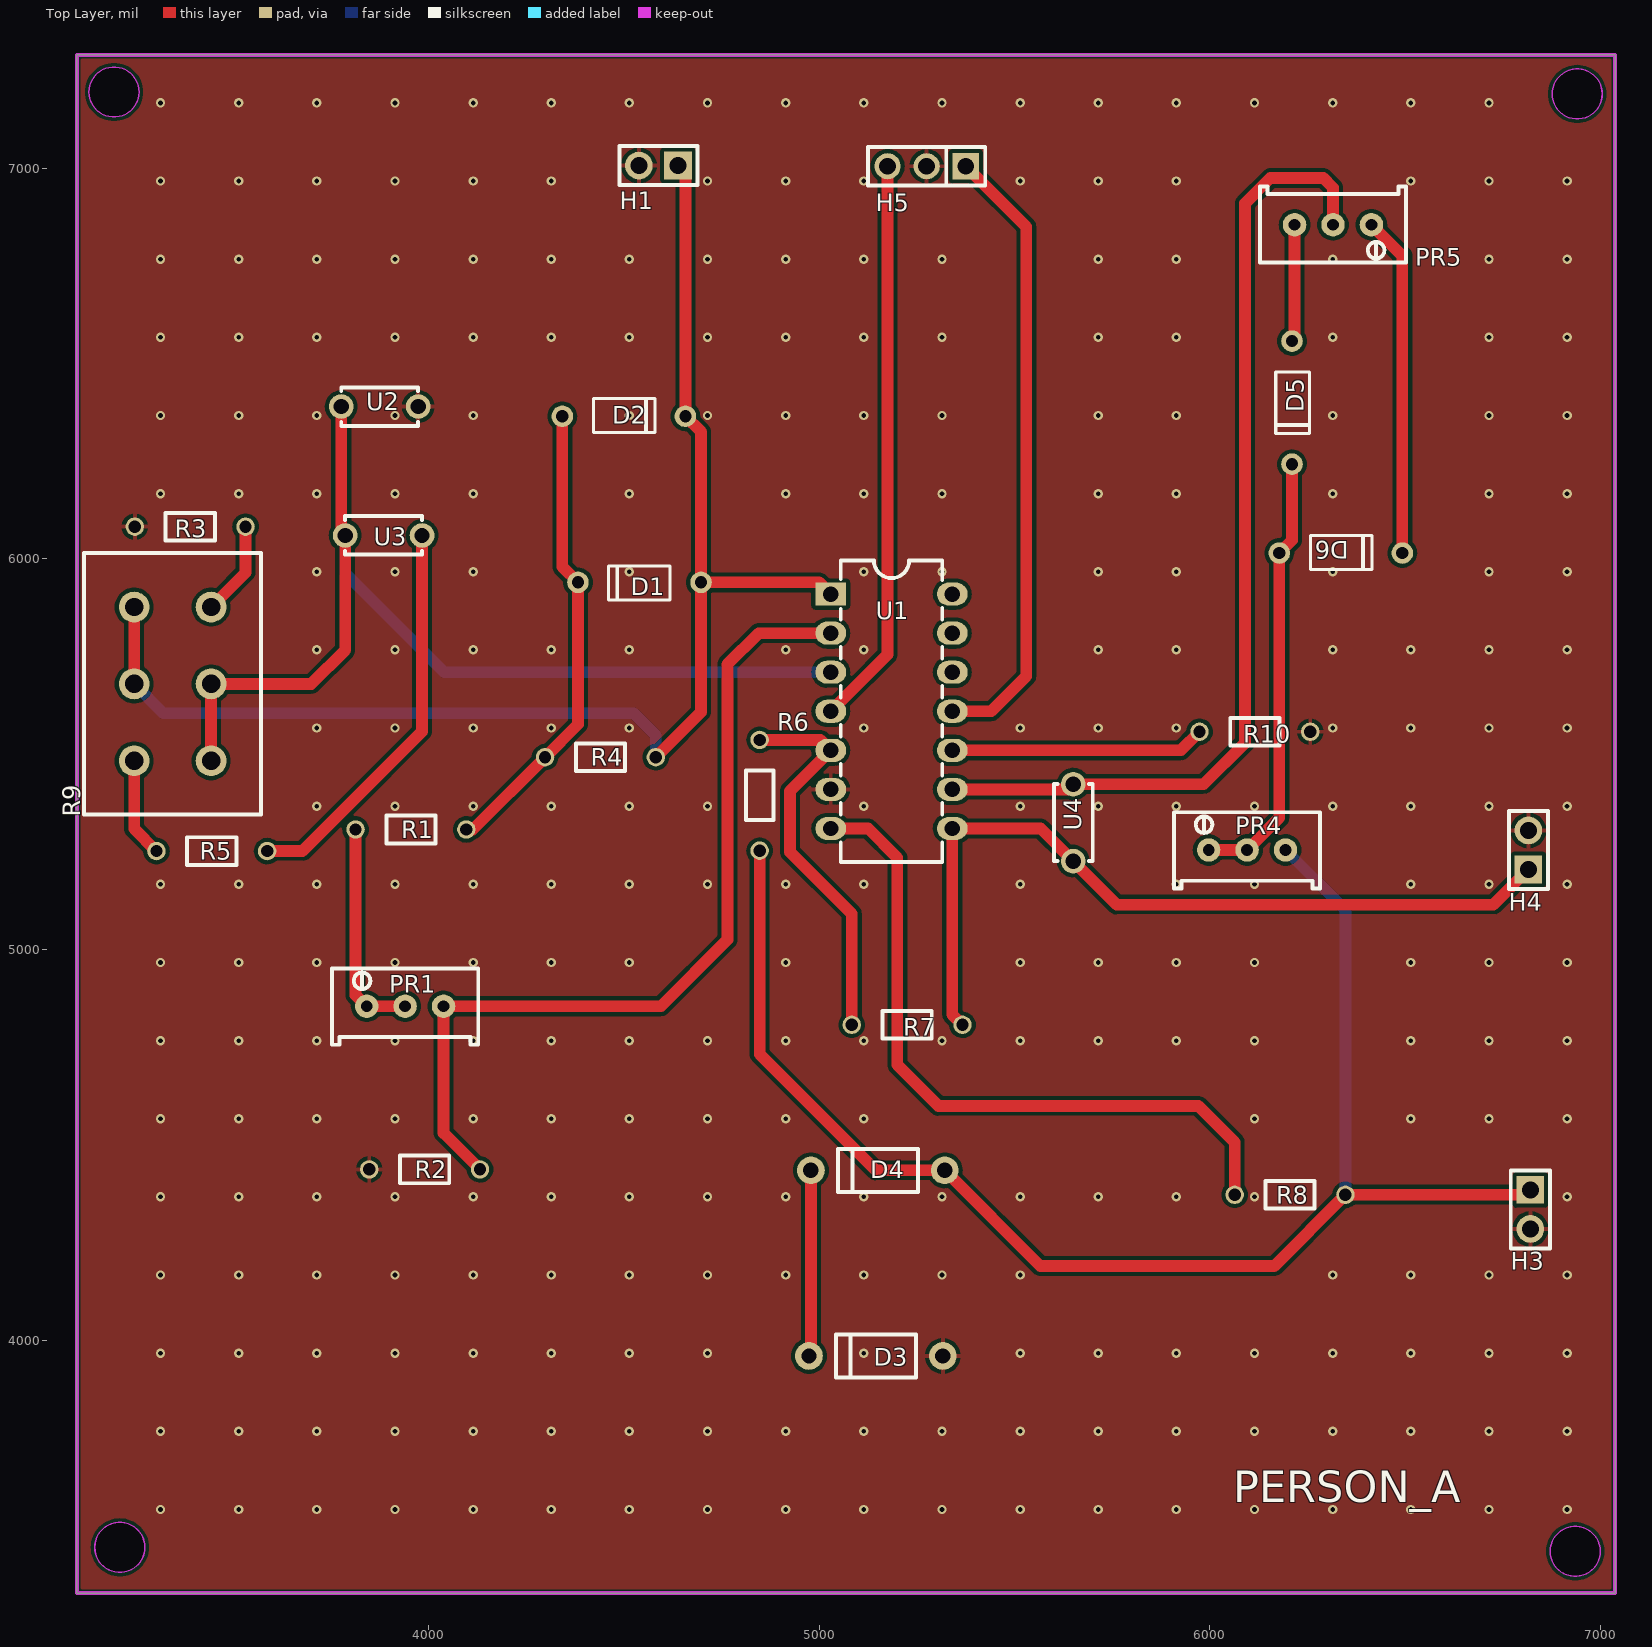
[diagram p0: Top Layer view]
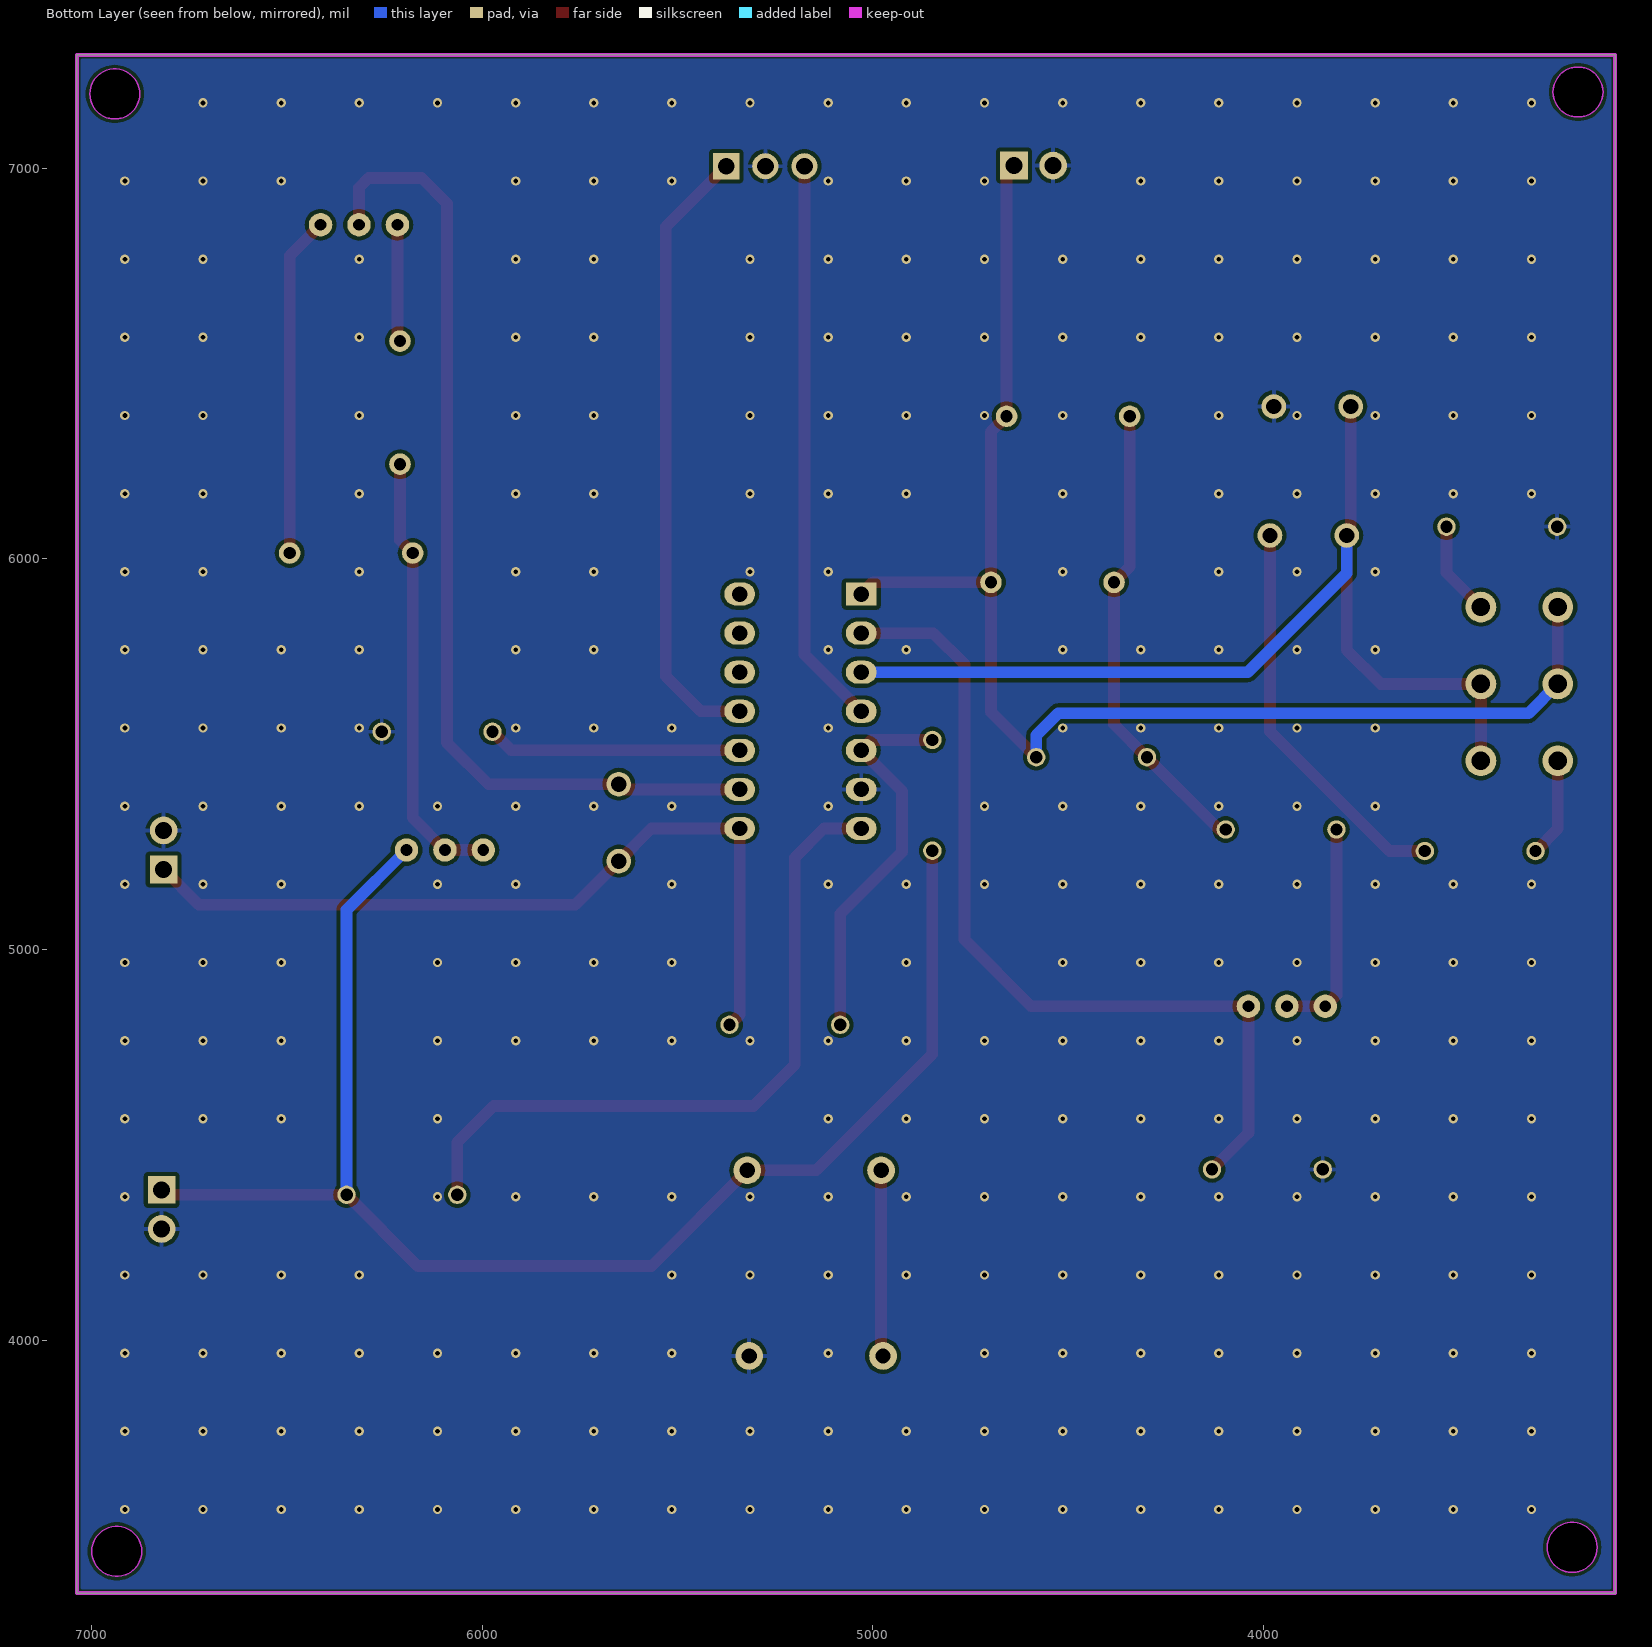
[diagram p1: Bottom Layer view, seen from below]
# Altium PCB MISC89085.pcbdoc
Units mil, origin at the board's own origin, x right, y up, seen from the top; angles counter-clockwise.
Board outline 3937.01 x 3937.01 mil, 2 copper layers (Top Layer, Bottom Layer), stack 62.206 mil thick; 27 components, 21 nets, 74 pads, 296 vias.

## Layer stack, top to bottom
Top Solder Mask Layer: solder mask 0.394, Dk 3.3
Top Layer: signal copper 1.379
Dielectric1: surface 59.449, FR4, Dk 4.5
Bottom Layer: signal copper 1.378
Bottom Solder Mask Layer: solder mask 0.394, Dk 3.3

## Board outline
3100,7290 3100,3352.99 7037.01,3352.99 7037.01,7290
cut-out: 3259.03,7195 cw(c3195,7195) 3130.97,7195 cw(c3195,7195)
cut-out: 7004.03,7190 cw(c6940,7190) 6875.97,7190 cw(c6940,7190)
cut-out: 6999.03,3460 cw(c6935,3460) 6870.97,3460 cw(c6935,3460)
cut-out: 3274.03,3470 cw(c3210,3470) 3145.97,3470 cw(c3210,3470)

## Design rules (kind name [scope] priority, off if disabled: settings)
BoardOutlineClearance copperThickness2oz_1 [All] p2 off: genericclearance=7.99 ignorepadtopadclearanceinfootprint=FALSE except(0: Arc-SplitContinuation Track-SplitContinuation SMDPad-SplitContinuation THPad-SplitContinuation Via-SplitContinuation Fill-SplitContinuation Region-SplitContinuation Poly-SplitContinuation Text-SplitContinuation Hole-SplitContinuation; 5.98: Arc-CutoutEdge SMDPad-CutoutEdge THPad-CutoutEdge Via-CutoutEdge Fill-CutoutEdge Region-CutoutEdge Text-CutoutEdge; 6.93: Hole-OutlineEdge Hole-CutoutEdge; 10: Poly-OutlineEdge Poly-CutoutEdge; 11.81: Arc-OutlineEdge Track-OutlineEdge SMDPad-OutlineEdge THPad-OutlineEdge Via-OutlineEdge Fill-OutlineEdge Region-OutlineEdge Text-OutlineEdge Track-CutoutEdge)
BoardOutlineClearance copperThickness1oz_1 [All] p4: genericclearance=4.02 ignorepadtopadclearanceinfootprint=FALSE except(0: Arc-SplitContinuation Track-SplitContinuation SMDPad-SplitContinuation THPad-SplitContinuation Via-SplitContinuation Fill-SplitContinuation Region-SplitContinuation Poly-SplitContinuation Text-SplitContinuation Hole-SplitContinuation; 6: SMDPad-CutoutEdge THPad-CutoutEdge Via-CutoutEdge Fill-CutoutEdge Region-CutoutEdge Text-CutoutEdge; 6.93: Hole-OutlineEdge Hole-CutoutEdge; 10: Poly-OutlineEdge Poly-CutoutEdge; 11.8: Arc-OutlineEdge Track-OutlineEdge SMDPad-OutlineEdge THPad-OutlineEdge Via-OutlineEdge Fill-OutlineEdge Region-OutlineEdge Text-OutlineEdge; 11.81: Arc-CutoutEdge Track-CutoutEdge)
Clearance copperThickness2oz [All] p1 off: gap=7.99 ignorepadtopadclearanceinfootprint=FALSE except(5.98: SMDPad-Track SMDPad-SMDPad THPad-Track SMDPad-THPad THPad-THPad Track-Via SMDPad-Via THPad-Via Via-Via Fill-Track Region-Track Fill-SMDPad Region-SMDPad Fill-THPad Region-THPad Fill-Via Region-Via Fill-Fill Fill-Region Region-Region Arc-Track Arc-SMDPad Arc-THPad Arc-Via Fill-Arc Region-Arc Arc-Arc Text-Track SMDPad-Text Text-THPad Text-Via Fill-Text Region-Text Arc-Text Text-Text; 6.93: Hole-Track Hole-SMDPad Hole-THPad Hole-Via Fill-Hole Region-Hole Hole-Arc Hole-Text; 10: Poly-Track Poly-SMDPad Poly-THPad Poly-Via Poly-Fill Poly-Region Poly-Poly Poly-Arc Poly-Text Poly-Hole)
Clearance copperThickness1oz [All] p3: gap=4.02 ignorepadtopadclearanceinfootprint=FALSE except(5.98: SMDPad-Track SMDPad-SMDPad THPad-Track SMDPad-THPad THPad-THPad Track-Via SMDPad-Via THPad-Via Via-Via Fill-Track Region-Track Fill-SMDPad Region-SMDPad Fill-THPad Region-THPad Fill-Via Region-Via Fill-Fill Fill-Region Region-Region; 6: Arc-Track Arc-SMDPad Arc-THPad Arc-Via Fill-Arc Region-Arc Arc-Arc Text-Track SMDPad-Text Text-THPad Text-Via Fill-Text Region-Text Arc-Text Text-Text; 6.93: Hole-Track Hole-SMDPad Hole-THPad Hole-Via Fill-Hole Region-Hole Hole-Arc Hole-Text; 10: Poly-Track Poly-SMDPad Poly-THPad Poly-Via Poly-Fill Poly-Region Poly-Poly Poly-Arc Poly-Text Poly-Hole)
Creepage creepage [All] p1: checkdistance=0 ignoreinternallayers=TRUE applytopolygonpour=TRUE
DiffPairsRouting differentialPair [All] p1: maxlimit=6 minlimit=6 mostfreqgap=6 toplayer_minwidth=5 toplayer_prefwidth=10 toplayer_maxwidth=100 toplayer_mingap=6 toplayer_prefgap=6 toplayer_maxgap=6 bottomlayer_minwidth=5 bottomlayer_prefwidth=10 bottomlayer_maxwidth=100 bottomlayer_mingap=6 bottomlayer_prefgap=6 bottomlayer_maxgap=6 maxuncoupledlength=10
HoleToHoleClearance otherClearance [All] p1: gap=11.81 allowstackedmicrovias=TRUE
Length netLength [All] p1: minlimit=0 maxlimit=0
MatchedLengths netLengthTolerance [All] p1: tolerance=1000
PasteMaskExpansion pasteMaskExpansion [All] p1: expansion=0
PlaneConnect innerPlane [All] p1: planeconnectstyle=Relief reliefexpansion=20 reliefentries=4 reliefconductorwidth=10 reliefairgap=10
PolygonConnect copperRegion [(InNet('GND'))] p1: connectstyle=Relief reliefconductorwidth=10 reliefentries=4 polygonreliefangle="90 Angle" airgapwidth=10 via.connectstyle=Relief via.reliefconductorwidth=10 via.reliefentries=4 via.polygonreliefangle="90 Angle" via.airgapwidth=10
RoutingVias viaSize [All] p1: holewidth=12.01 width=24.02 viastyle="Through Hole" minholewidth=11.81 minwidth=19.68 maxholewidth=248.03 maxwidth=393.7
SolderMaskExpansion solderMaskExpansion [IsVia] p1: expansion=-1000 istentingtop=TRUE
SolderMaskExpansion solderMaskExpansion [All] p2: expansion=2 istentingtop=FALSE
Width copperThickness2oz_2 [All] p1 off: maxlimit=100 minlimit=8 preferedwidth=10
Width copperThickness1oz_2 [All] p2: maxlimit=100 minlimit=5 preferedwidth=10

## Components (designator, comment, footprint, x,y, rotation, side; value= is the part's Value field where it differs from the comment)
D1 "1N4148" DO-35_BD2.2-L4.0-D0.50_1N4148 4540,5940 r180 top
D2 "1N4148" DO-35_BD2.2-L4.0-D0.50_1N4148 4500,6365 r0 top
D3 "1N4731A" DO-41_BD2.4-L4.7-P8.70-D0.9-RD 5145,3960 r0 top
D4 "1N4731A" DO-41_BD2.4-L4.7-P8.70-D0.9-RD 5150,4435 r0 top
D5 "1N4148" DO-35_BD2.2-L4.0-D0.50_1N4148 6210,6400 r270 top
D6 "1N4148" DO-35_BD2.2-L4.0-D0.50_1N4148 6335,6015 r0 top
H1 "" HDR-TH_2P-P2.54-V-M-1 4588.39,7006.69 r180 top
H3 "" HDR-TH_2P-P2.54-V-M-1 6820,4335 r270 top
H4 "" HDR-TH_2P-P2.54-V-M-1 6815,5255 r90 top
H5 "" HDR-TH_3P-P2.54-V-M 5275,7005 r180 top
PR1 "10kΩ" R_3296 3940,4860 r0 top
PR4 "10kΩ" R_3296 6095,5260 r0 top
PR5 "10kΩ" R_3296 6315,6850 r180 top
R1 "5.1kΩ" Res_1/8W 3955,5305 r0 top
R2 "5.1kΩ" Res_1/8W 3990,4435 r0 top
R3 "600Ω" Res_1/8W 3390,6080 r0 top
R4 "2kΩ" Res_1/8W 4440,5490 r0 top
R5 "600Ω" Res_1/8W 3445.3,5254.62 r180 top
R6 "10kΩ" Res_1/8W 4845,5395 r270 top
R7 "20kΩ" Res_1/8W 5225,4805 r0 top
R8 "100Ω" Res_1/8W 6205,4370 r0 top
R9 "" WH148 3345,5680 r90 top
R10 "10KΩ" Res_1/8W 6115,5560 r180 top
U1 "LF347BN/PB" PDIP-14_L19.6-W6.5-P2.54-LS7.9-BL 5185,5610 r270 top
U2 "47nF" CAP-TH_L5.0-W2.5-P5.00-D1.0 3875,6390 r0 top
U3 "47nF" CAP-TH_L5.0-W2.5-P5.00-D1.0 3885,6060 r180 top
U4 "100nF" CAP-TH_L5.0-W2.5-P5.00-D1.0 5650,5325 r90 top

## Footprints (in the part's own frame and the unit in brackets; to place one, negate y for a bottom-side part, rotate by r counter-clockwise, add the part's x,y. Pads: shape width x height; smd on the part's side, far side on the other; paste and mask are expansions set on the pad)
CAP-TH_L5.0-W2.5-P5.00-D1.0 [mm]
  round 1.6 hole 1: 1(-2.5,0) 2(2.5,0)
  silkscreen extent -2.5,-1.27 2.5,1.25
DO-35_BD2.2-L4.0-D0.50_1N4148 [mm]
  round 1.4 hole 0.8 paste+0 mask+0.05: 1(-4,0) 2(4,0)
  silkscreen extent -1.98,-1.06 2.02,1.14
DO-41_BD2.4-L4.7-P8.70-D0.9-RD [mm]
  round 1.8 hole 1: 1(-4.35,0) 2(4.35,0)
  silkscreen extent -2.6,-1.4 2.6,1.4
HDR-TH_2P-P2.54-V-M-1 [mm]
  rect 1.8x1.8 hole 1.1: 1(-1.27,0)
  round 1.8 hole 1.1: 2(1.27,0)
  silkscreen extent -2.54,-1.27 2.54,1.27
HDR-TH_3P-P2.54-V-M [mm]
  rect 1.7x1.7 hole 1.1: 1(-2.54,0)
  round 1.7 hole 1.1: 2(0,0) 3(2.54,0)
  silkscreen extent -3.81,-1.25 3.81,1.25
PDIP-14_L19.6-W6.5-P2.54-LS7.9-BL [mm]
  rect 1.5x2 hole 1: 1(-7.62,-3.95)
  oval 1.5x2 hole 1: 2(-5.08,-3.95) 3(-2.54,-3.95) 4(0,-3.95) 5(2.54,-3.95) 6(5.08,-3.95) 7(7.62,-3.95) 8(7.62,3.95) 9(5.08,3.95) 10(2.54,3.95) 11(0,3.95) 12(-2.54,3.95) 13(-5.08,3.95) 14(-7.62,3.95)
  silkscreen extent -9.8,-3.3 9.8,3.3
R_3296 [mil]
  round 60 hole 30 paste+0 mask+2: 1(-98.4,-5) 2(0,-5) 3(98.4,-5)
  silkscreen extent -187,-103 187,92
Res_1/8W [mil]
  round 47.2 hole 31.5 paste+0 mask+2: 1(-141.7,2.48) 2(141.7,2.48)
  silkscreen extent -63,-33 63,38
WH148 [mm]
  round 2 hole 1.2 paste+0 mask+0.102: 1(-5,-2.5) 2(0,-2.5) 3(5,-2.5) 4(-5,2.5) 5(0,2.5) 6(5,2.5)
  silkscreen extent -8.5,-5.75 8.5,5.75

## Via types
v1: diameter 24.02, hole 12, Top Layer to Bottom Layer, 296 vias

## Nets (pads, with @x,y where several pads share a name; then routed paths per layer and width w, separated by ;. In a path a pad name is that pad's centre, name@x,y a point inside that pad or via, vN(x,y) a via of type N, cw(c..) or ccw(c..) an arc to the next point about the centre after c; other vN are vias at no path point)
12V: H5.3 U1.4 | length 1455.3
  Top Layer w30: U1.4 5175,5755.51 H5.3
$1N1: PR1.1 PR1.2 R1.1 | length 562.6
  Top Layer w30: R1.1 3813.3,4883.3 PR1.1 PR1.2
$1N2: PR1.3 R2.2 U1.2 | length 2255.8
  Top Layer w30: R2.2 4038.4,4530.78 PR1.3 4595,4855 4765,5025 4765,5730 4845,5810 U1.2
$1N7: R9.1 R9.2 U1.3 U2.1 U3.2 | length 2647.9
  Top Layer w30: R9.1 R9.2 3700,5680 3786.57,5766.57 U3.2 3776.57,6070 U2.1
  Bottom Layer w30: U3.2 3786.57,5963.43 4040,5710 U1.3
$1N10: D1.2 D2.1 R1.2 R4.1 | length 1202.2
  Top Layer w30: R1.2 4113.3,5307.48 R4.1 4382.52,5576.7 D1.2 4342.52,5980 D2.1
$1N11: D1.1 D2.2 H1.1 R4.2 R9.5 R9.6 U1.1 | length 3573.4
  Top Layer w30: R9.5 R9.6 ; R4.2 4697.48,5608.26 D1.1 ; H1.1 4657.48,6987.6 D2.2 4697.48,6325 D1.1 ; U1.1 4999.49,5940 D1.1
  Bottom Layer w30: R9.5 3321.57,5605 4525,5605 4581.7,5548.3 R4.2
$1N12: R5.1 U3.1 | length 1024.9
  Top Layer w30: R5.1 3677.15,5252.15 3983.43,5558.43 U3.1
$1N16: R6.1 R7.1 U1.5 | length 1004.4
  Top Layer w30: R6.1 5002.79,5536.7 U1.5 4925,5405.51 4925,5250 5083.3,5091.7 R7.1
$1N19: D3.1 D4.1 | length 477.1
  Top Layer w30: D3.1 4978.74,3965 D4.1
$1N26: H4.1 R7.2 U1.8 U4.1 | length 2105.9
  Top Layer w30: R7.2 5340.51,4833.67 U1.8 5566.57,5310 U4.1 5761.57,5115 6725,5115 H4.1
$1N27: R10.2 U1.10 | length 652.5
  Top Layer w30: U1.10 5925.78,5510 R10.2
$1N37: R8.1 U1.7 | length 1811.2
  Top Layer w30: U1.7 5125,5310 5200,5235 5200,4705 5305,4600 5970,4600 6063.3,4506.7 R8.1
$1N39: D4.2 H3.1 PR4.3 R6.2 R8.2 | length 3744.8
  Top Layer w30: R6.2 4847.48,4732.52 5145,4435 D4.2 5566.26,4190 6164.22,4190 R8.2 6807.48,4372.48 H3.1
  Bottom Layer w30: PR4.3 6346.7,5101.7 R8.2
$1N40: PR5.2 U1.9 U4.2 | length 2536.5
  Top Layer w30: U1.9 5636.58,5410 U4.2 5983.43,5423.43 6090,5530 6090,6910 6155,6975 6290,6975 6315,6950 PR5.2
$1N41: D5.2 D6.1 PR4.1 PR4.2 | length 1133.6
  Top Layer w30: PR4.1 PR4.2 6177.52,5337.52 D6.1 6210,6047.48 D5.2
$1N42: D5.1 PR5.3 | length 300.3
  Top Layer w30: D5.1 6216.6,6564.08 PR5.3
$1N43: D6.2 PR5.1 | length 872.8
  Top Layer w30: PR5.1 6492.48,6775.92 D6.2
$1N46: R3.2 R9.3 | length 242.2
  Top Layer w30: R9.3 3531.7,5965.12 R3.2
$1N47: R5.2 R9.4 | length 254.6
  Top Layer w30: R9.4 3246.57,5309.17 R5.2
-12V: H5.1 U1.11 | length 1596
  Top Layer w30: U1.11 5440,5610 5530,5700 5530,6850 H5.1
GND: D3.2 H1.2 H3.2 H4.2 H5.2 R2.1 R3.1 R10.1 U1.6 U2.2
  other v1: 3314.1,3567.09 3514.1,3567.09 3714.1,3567.09 3914.1,3567.09 4114.1,3567.09 4314.1,3567.09 4514.1,3567.09 4714.1,3567.09 4914.1,3567.09 5114.1,3567.09 5314.1,3567.09 5514.1,3567.09 5714.1,3567.09 5914.1,3567.09 6114.1,3567.09 6314.1,3567.09 6514.1,3567.09 6714.1,3567.09 6914.1,3567.09 3314.1,3767.09 3514.1,3767.09 3714.1,3767.09 3914.1,3767.09 4114.1,3767.09 4314.1,3767.09 4514.1,3767.09 4714.1,3767.09 4914.1,3767.09 5114.1,3767.09 5314.1,3767.09 5514.1,3767.09 5714.1,3767.09 5914.1,3767.09 6114.1,3767.09 6314.1,3767.09 6514.1,3767.09 6714.1,3767.09 6914.1,3767.09 3314.1,3967.09 3514.1,3967.09 3714.1,3967.09 3914.1,3967.09 4114.1,3967.09 4314.1,3967.09 4514.1,3967.09 4714.1,3967.09 5114.1,3967.09 5514.1,3967.09 5714.1,3967.09 5914.1,3967.09 6114.1,3967.09 6314.1,3967.09 6514.1,3967.09 6714.1,3967.09 6914.1,3967.09 3314.1,4167.09 3514.1,4167.09 3714.1,4167.09 3914.1,4167.09 4114.1,4167.09 4314.1,4167.09 4514.1,4167.09 4714.1,4167.09 4914.1,4167.09 5114.1,4167.09 5314.1,4167.09 5514.1,4167.09 6314.1,4167.09 6514.1,4167.09 6714.1,4167.09 6914.1,4167.09 3314.1,4367.09 3514.1,4367.09 3714.1,4367.09 3914.1,4367.09 4114.1,4367.09 4314.1,4367.09 4514.1,4367.09 4714.1,4367.09 4914.1,4367.09 5114.1,4367.09 5314.1,4367.09 5514.1,4367.09 5714.1,4367.09 5914.1,4367.09 6114.1,4367.09 6914.1,4367.09 3314.1,4567.09 3514.1,4567.09 3714.1,4567.09 3914.1,4567.09 4114.1,4567.09 4314.1,4567.09 4514.1,4567.09 4714.1,4567.09 4914.1,4567.09 5114.1,4567.09 6114.1,4567.09 6514.1,4567.09 6714.1,4567.09 6914.1,4567.09 3314.1,4767.09 3514.1,4767.09 3714.1,4767.09 3914.1,4767.09 4114.1,4767.09 4314.1,4767.09 4514.1,4767.09 4714.1,4767.09 4914.1,4767.09 5114.1,4767.09 5314.1,4767.09 5514.1,4767.09 5714.1,4767.09 5914.1,4767.09 6114.1,4767.09 6514.1,4767.09 6714.1,4767.09 6914.1,4767.09 3314.1,4967.09 3514.1,4967.09 3714.1,4967.09 3914.1,4967.09 4114.1,4967.09 4314.1,4967.09 4514.1,4967.09 4914.1,4967.09 5514.1,4967.09 5714.1,4967.09 5914.1,4967.09 6114.1,4967.09 6514.1,4967.09 6714.1,4967.09 6914.1,4967.09 3314.1,5167.09 3514.1,5167.09 3714.1,5167.09 3914.1,5167.09 4114.1,5167.09 4314.1,5167.09 4514.1,5167.09 4714.1,5167.09 4914.1,5167.09 5114.1,5167.09 5514.1,5167.09 5914.1,5167.09 6114.1,5167.09 6514.1,5167.09 6714.1,5167.09 6914.1,5167.09 3714.1,5367.09 3914.1,5367.09 4114.1,5367.09 4314.1,5367.09 4514.1,5367.09 4714.1,5367.09 5114.1,5367.09 5514.1,5367.09 5714.1,5367.09 5914.1,5367.09 6114.1,5367.09 6314.1,5367.09 6514.1,5367.09 6714.1,5367.09 6914.1,5367.09 3714.1,5567.09 3914.1,5567.09 4114.1,5567.09 4314.1,5567.09 4514.1,5567.09 5114.1,5567.09 5514.1,5567.09 5714.1,5567.09 5914.1,5567.09 6314.1,5567.09 6514.1,5567.09 6714.1,5567.09 6914.1,5567.09 3714.1,5767.09 3914.1,5767.09 4114.1,5767.09 4314.1,5767.09 4514.1,5767.09 4914.1,5767.09 5114.1,5767.09 5714.1,5767.09 5914.1,5767.09 6314.1,5767.09 6514.1,5767.09 6714.1,5767.09 6914.1,5767.09 3714.1,5967.09 3914.1,5967.09 4114.1,5967.09 4514.1,5967.09 5114.1,5967.09 5314.1,5967.09 5714.1,5967.09 5914.1,5967.09 6314.1,5967.09 6714.1,5967.09 6914.1,5967.09 3314.1,6167.09 3514.1,6167.09 3714.1,6167.09 3914.1,6167.09 4114.1,6167.09 4514.1,6167.09 4914.1,6167.09 5114.1,6167.09 5314.1,6167.09 5714.1,6167.09 5914.1,6167.09 6314.1,6167.09 6714.1,6167.09 6914.1,6167.09 3314.1,6367.09 3514.1,6367.09 3714.1,6367.09 3914.1,6367.09 4114.1,6367.09 4514.1,6367.09 4714.1,6367.09 4914.1,6367.09 5114.1,6367.09 5314.1,6367.09 5714.1,6367.09 5914.1,6367.09 6314.1,6367.09 6714.1,6367.09 6914.1,6367.09 3314.1,6567.09 3514.1,6567.09 3714.1,6567.09 3914.1,6567.09 4114.1,6567.09 4314.1,6567.09 4514.1,6567.09 4714.1,6567.09 4914.1,6567.09 5114.1,6567.09 5314.1,6567.09 5714.1,6567.09 5914.1,6567.09 6314.1,6567.09 6714.1,6567.09 6914.1,6567.09 3314.1,6767.09 3514.1,6767.09 3714.1,6767.09 3914.1,6767.09 4114.1,6767.09 4314.1,6767.09 4514.1,6767.09 4714.1,6767.09 4914.1,6767.09 5114.1,6767.09 5314.1,6767.09 5714.1,6767.09 5914.1,6767.09 6314.1,6767.09 6714.1,6767.09 6914.1,6767.09 3314.1,6967.09 3514.1,6967.09 3714.1,6967.09 3914.1,6967.09 4114.1,6967.09 4314.1,6967.09 4714.1,6967.09 4914.1,6967.09 5114.1,6967.09 5514.1,6967.09 5714.1,6967.09 5914.1,6967.09 6514.1,6967.09 6714.1,6967.09 6914.1,6967.09 3314.1,7167.09 3514.1,7167.09 3714.1,7167.09 3914.1,7167.09 4114.1,7167.09 4314.1,7167.09 4514.1,7167.09 4714.1,7167.09 4914.1,7167.09 5114.1,7167.09 5314.1,7167.09 5514.1,7167.09 5714.1,7167.09 5914.1,7167.09 6114.1,7167.09 6314.1,7167.09 6514.1,7167.09 6714.1,7167.09
pads on no net: U1.12 U1.13 U1.14

## Polygon pours and split planes (outlines as drawn)
GND on Top Layer (solid, remove dead copper, pour order 0): 3000,7410 3000,3170 7385,3170 7385,7410
GND on Bottom Layer (solid, remove dead copper, pour order 2): 3035,7340 3035,3000 7425,3000 7425,7340

## Keep-outs
Board Outline Layer:
  region: 3259.03,7195 cw(c3195,7195) 3130.97,7195 cw(c3195,7195)
  circle w0.1: c3195,7195 r64.03
  region: 3259.03,7195 3258.66,7188.08 3257.53,7181.24 3255.68,7174.55 3253.11,7168.11 3249.87,7161.99 3245.97,7156.25 3241.49,7150.97 3236.45,7146.2 3230.93,7142 3224.99,7138.43 3218.7,7135.52 3212.13,7133.3 3205.36,7131.81 3198.47,7131.06 3191.53,7131.06 3184.64,7131.81 3177.87,7133.3 3171.3,7135.52 3165.01,7138.43 3159.07,7142 3153.55,7146.2 3148.51,7150.97 3144.03,7156.25 3140.13,7161.99 3136.89,7168.11 3134.32,7174.55 3132.47,7181.24 3131.34,7188.08 3130.97,7195 3131.34,7201.92 3132.47,7208.76 3134.32,7215.45 3136.89,7221.89 3140.13,7228.01 3144.03,7233.75 3148.51,7239.03 3153.55,7243.8 3159.07,7248 3165.01,7251.57 3171.3,7254.48 3177.87,7256.7 3184.64,7258.19 3191.53,7258.94 3198.47,7258.94 3205.36,7258.19 3212.13,7256.7 3218.7,7254.48 3224.99,7251.57 3230.93,7248 3236.45,7243.8 3241.49,7239.03 3245.97,7233.75 3249.87,7228.01 3253.11,7221.89 3255.68,7215.45 3257.53,7208.76 3258.66,7201.92
  region: 7004.03,7190 cw(c6940,7190) 6875.97,7190 cw(c6940,7190)
  circle w0.1: c6940,7190 r64.03
  region: 7004.03,7190 7003.66,7183.08 7002.53,7176.24 7000.68,7169.55 6998.11,7163.11 6994.87,7156.99 6990.97,7151.25 6986.49,7145.97 6981.45,7141.2 6975.93,7137 6969.99,7133.43 6963.7,7130.52 6957.13,7128.3 6950.36,7126.81 6943.47,7126.06 6936.53,7126.06 6929.64,7126.81 6922.87,7128.3 6916.3,7130.52 6910.01,7133.43 6904.07,7137 6898.55,7141.2 6893.51,7145.97 6889.03,7151.25 6885.13,7156.99 6881.89,7163.11 6879.32,7169.55 6877.47,7176.24 6876.34,7183.08 6875.97,7190 6876.34,7196.92 6877.47,7203.76 6879.32,7210.45 6881.89,7216.89 6885.13,7223.01 6889.03,7228.75 6893.51,7234.03 6898.55,7238.8 6904.07,7243 6910.01,7246.57 6916.3,7249.48 6922.87,7251.7 6929.64,7253.19 6936.53,7253.94 6943.47,7253.94 6950.36,7253.19 6957.13,7251.7 6963.7,7249.48 6969.99,7246.57 6975.93,7243 6981.45,7238.8 6986.49,7234.03 6990.97,7228.75 6994.87,7223.01 6998.11,7216.89 7000.68,7210.45 7002.53,7203.76 7003.66,7196.92
  region: 6999.03,3460 cw(c6935,3460) 6870.97,3460 cw(c6935,3460)
  circle w0.1: c6935,3460 r64.03
  region: 6999.03,3460 6998.66,3453.08 6997.53,3446.24 6995.68,3439.55 6993.11,3433.11 6989.87,3426.99 6985.97,3421.25 6981.49,3415.97 6976.45,3411.2 6970.93,3407 6964.99,3403.43 6958.7,3400.52 6952.13,3398.3 6945.36,3396.81 6938.47,3396.06 6931.53,3396.06 6924.64,3396.81 6917.87,3398.3 6911.3,3400.52 6905.01,3403.43 6899.07,3407 6893.55,3411.2 6888.51,3415.97 6884.03,3421.25 6880.13,3426.99 6876.89,3433.11 6874.32,3439.55 6872.47,3446.24 6871.34,3453.08 6870.97,3460 6871.34,3466.92 6872.47,3473.76 6874.32,3480.45 6876.89,3486.89 6880.13,3493.01 6884.03,3498.75 6888.51,3504.03 6893.55,3508.8 6899.07,3513 6905.01,3516.57 6911.3,3519.48 6917.87,3521.7 6924.64,3523.19 6931.53,3523.94 6938.47,3523.94 6945.36,3523.19 6952.13,3521.7 6958.7,3519.48 6964.99,3516.57 6970.93,3513 6976.45,3508.8 6981.49,3504.03 6985.97,3498.75 6989.87,3493.01 6993.11,3486.89 6995.68,3480.45 6997.53,3473.76 6998.66,3466.92
  region: 3274.03,3470 cw(c3210,3470) 3145.97,3470 cw(c3210,3470)
  circle w0.1: c3210,3470 r64.03
  region: 3274.03,3470 3273.66,3463.08 3272.53,3456.24 3270.68,3449.55 3268.11,3443.11 3264.87,3436.99 3260.97,3431.25 3256.49,3425.97 3251.45,3421.2 3245.93,3417 3239.99,3413.43 3233.7,3410.52 3227.13,3408.3 3220.36,3406.81 3213.47,3406.06 3206.53,3406.06 3199.64,3406.81 3192.87,3408.3 3186.3,3410.52 3180.01,3413.43 3174.07,3417 3168.55,3421.2 3163.51,3425.97 3159.03,3431.25 3155.13,3436.99 3151.89,3443.11 3149.32,3449.55 3147.47,3456.24 3146.34,3463.08 3145.97,3470 3146.34,3476.92 3147.47,3483.76 3149.32,3490.45 3151.89,3496.89 3155.13,3503.01 3159.03,3508.75 3163.51,3514.03 3168.55,3518.8 3174.07,3523 3180.01,3526.57 3186.3,3529.48 3192.87,3531.7 3199.64,3533.19 3206.53,3533.94 3213.47,3533.94 3220.36,3533.19 3227.13,3531.7 3233.7,3529.48 3239.99,3526.57 3245.93,3523 3251.45,3518.8 3256.49,3514.03 3260.97,3508.75 3264.87,3503.01 3268.11,3496.89 3270.68,3490.45 3272.53,3483.76 3273.66,3476.92
  lines w10: 3100,3352.99 3100,7290 7037.01,7290 7037.01,3352.99 3100,3352.99

## Silkscreen, mask and mechanical layers (free items; w line width, h text height)
Top Silkscreen Layer:
  text "PERSON_A" at 6060,3585 h80
Mechanical Layer:
  circle w0.1: c3195,7195 r64.03
  circle w0.1: c6940,7190 r64.03
  circle w0.1: c6935,3460 r64.03
  circle w0.1: c3210,3470 r64.03